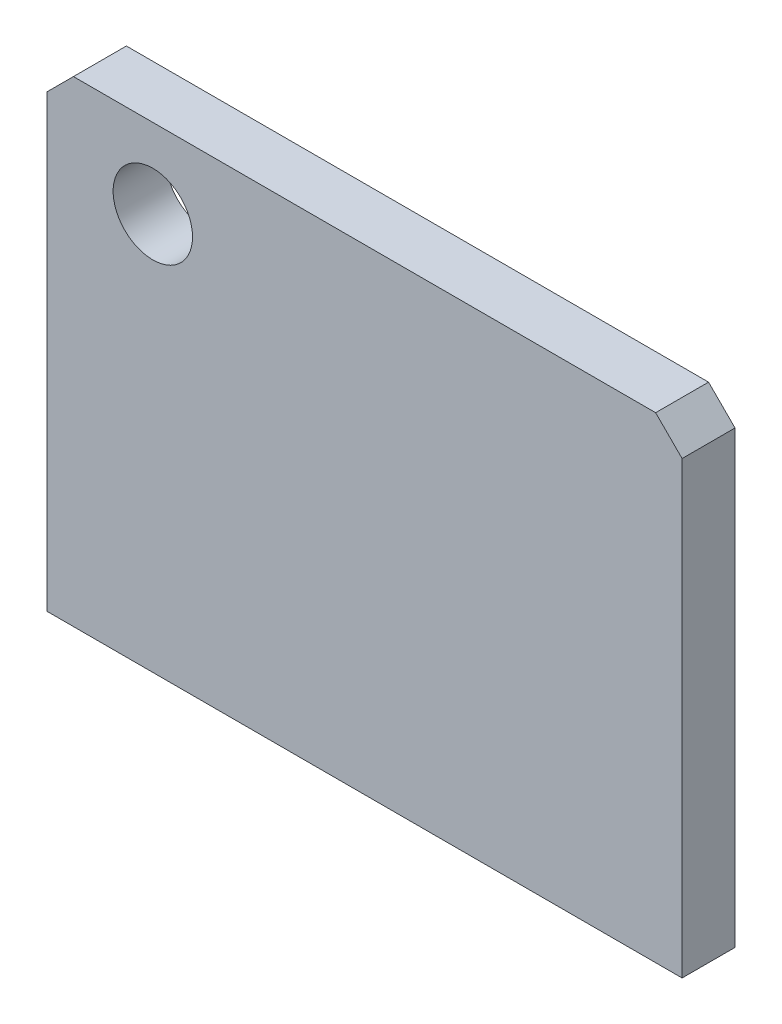
SolidWorks part; units mm, degrees
material "1023 Carbon Steel Plate (SS)"
ref_plane "Front Plane" through (0, 0, 0) normal (0, 0, 1) x (1, 0, 0)
ref_plane "Top Plane" through (0, 0, 0) normal (0, 1, 0) x (1, 0, 0)
ref_plane "Right Plane" through (0, 0, 0) normal (1, 0, 0) x (0, 0, -1)
sketch "Sketch1" plane through (0, 0, 0) normal (0, 0, 1) x (1, 0, 0)
  line L1 (60, 45) -> (-60, 45)
  line L2 (60, 45) -> (60, -45)
  line L3 (60, -45) -> (-60, -45)
  line L4 (-60, 45) -> (-60, -45)
  line L5 (60, 45) -> (-60, -45) construction
  line L6 (60, -45) -> (-60, 45) construction
  point P0 (0, 0)
  dimension "D1" = 120
  dimension "D2" = 90
extrude "Boss-Extrude1" add sketch "Sketch1" along normal blind 10
sketch "Sketch2" plane through (0, 0, 10) normal (0, 0, 1) x (1, 0, 0)
  line L0 (-60, 45) -> (-60, -45) construction
  line L1 (60, 45) -> (-60, 45) construction
  circle A0 centre (-40, 30) radius 7.5
  dimension "D1" = 15
  dimension "D2" = 20
  dimension "D3" = 15
extrude "Cut-Extrude1" cut sketch "Sketch2" against normal blind 10
chamfer "Chamfer1" distance 5 angle 45 2 edges at (60, 45, 5) (-60, 45, 5)
